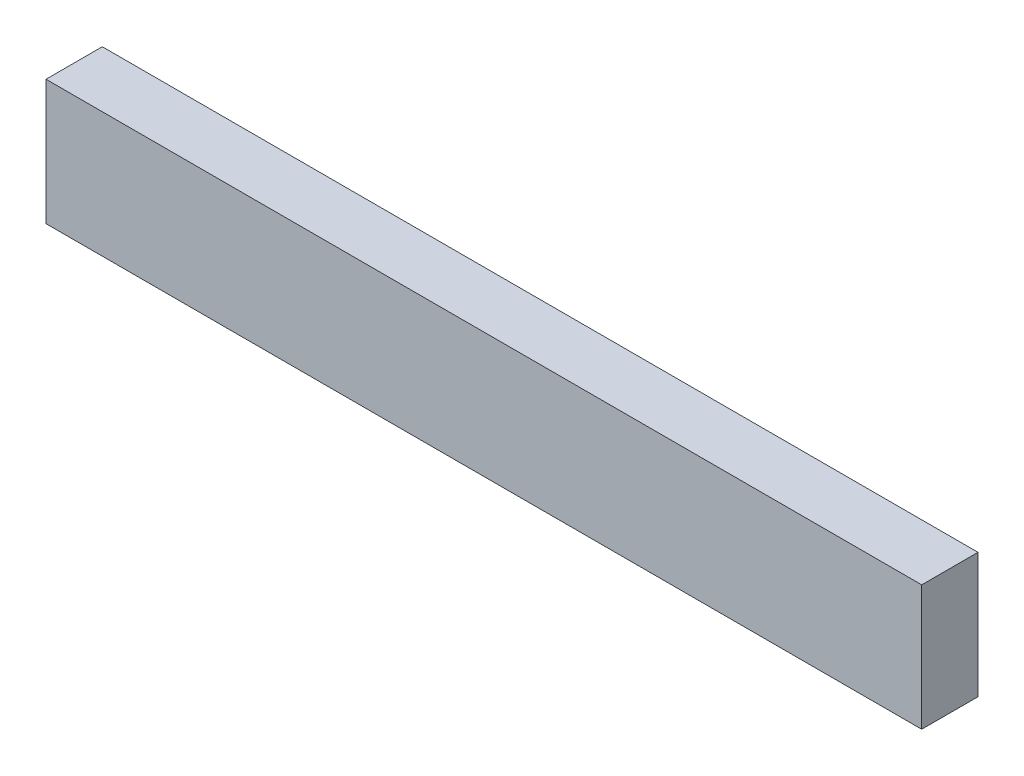
from build123d import *

# Parameters (mm, degrees)
SKETCH_1_W      = 140
SKETCH_1_H      = 20
EXTRUDE_1_DEPTH = 9


with BuildPart() as part:
    # 草图1 → 凸台-拉伸1 (new body)
    with BuildSketch(Plane.XY):
        Rectangle(SKETCH_1_W, SKETCH_1_H)
    extrude(amount=EXTRUDE_1_DEPTH)


solid = part.part
